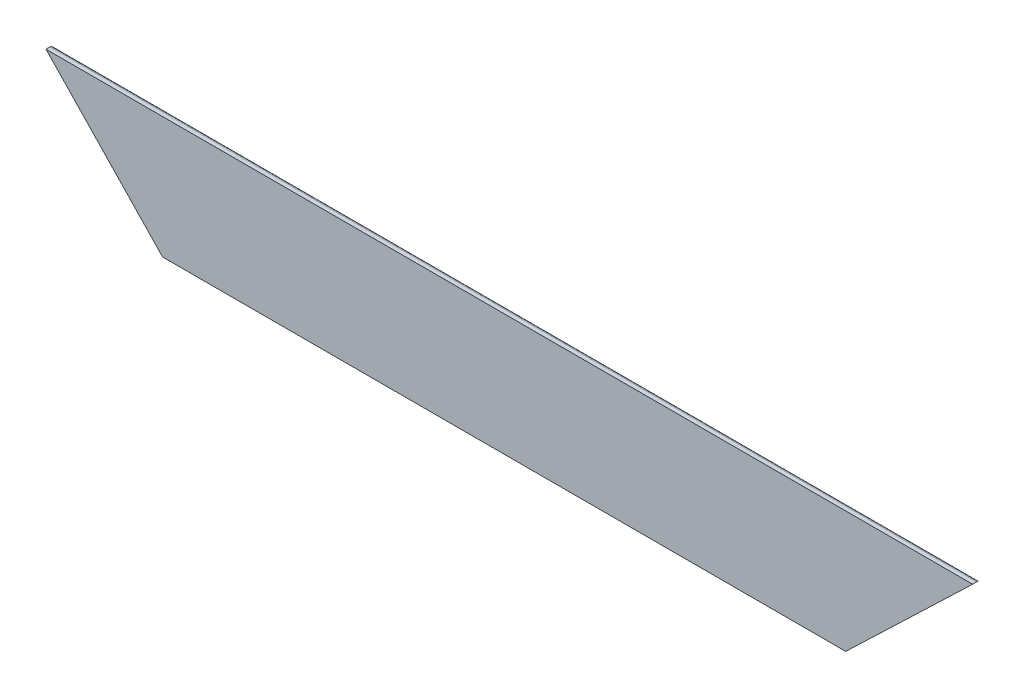
from build123d import *

# Parameters (mm, degrees)
EXTRUDE1_DEPTH    = 900
SKETCH2_OUTSIDE_W = 2163.11
SKETCH2_OUTSIDE_H = 463.11
EXTRUDE5_DEPTH    = 100


with BuildPart() as part:
    # Sketch1 → Extrude1 (new, symmetric)
    with BuildSketch(Plane(origin=(0, 0, 0), x_dir=(0, 0, -1), z_dir=(1, 0, 0))):
        with BuildLine():
            Line((-44, 47.3), (-44, -32))
            ThreePointArc((-44, -32), (-40.485281374, -40.485281374), (-32, -44))
            Line((-32, -44), (47.3, -44))
            ThreePointArc((47.3, -44), (49.209188309, -44.790811691), (50, -46.7))
            Line((50, -46.7), (50, -50))
            Line((50, -50), (-50, -50))
            Line((-50, -50), (-50, 50))
            Line((-50, 50), (-46.7, 50))
            ThreePointArc((-46.7, 50), (-44.790811691, 49.209188309), (-44, 47.3))
        make_face()
    extrude(amount=EXTRUDE1_DEPTH, both=True)

    # Sketch2 outside → Extrude5 (cut)
    with BuildSketch(Plane.XY.offset(50)):
        Rectangle(SKETCH2_OUTSIDE_W, SKETCH2_OUTSIDE_H)
        Polygon((-138.272358385, 50), (-900, 50), (-535.395927853, -330.516583835), align=None, mode=Mode.SUBTRACT)
    extrude(amount=-EXTRUDE5_DEPTH, mode=Mode.SUBTRACT)


solid = part.part
